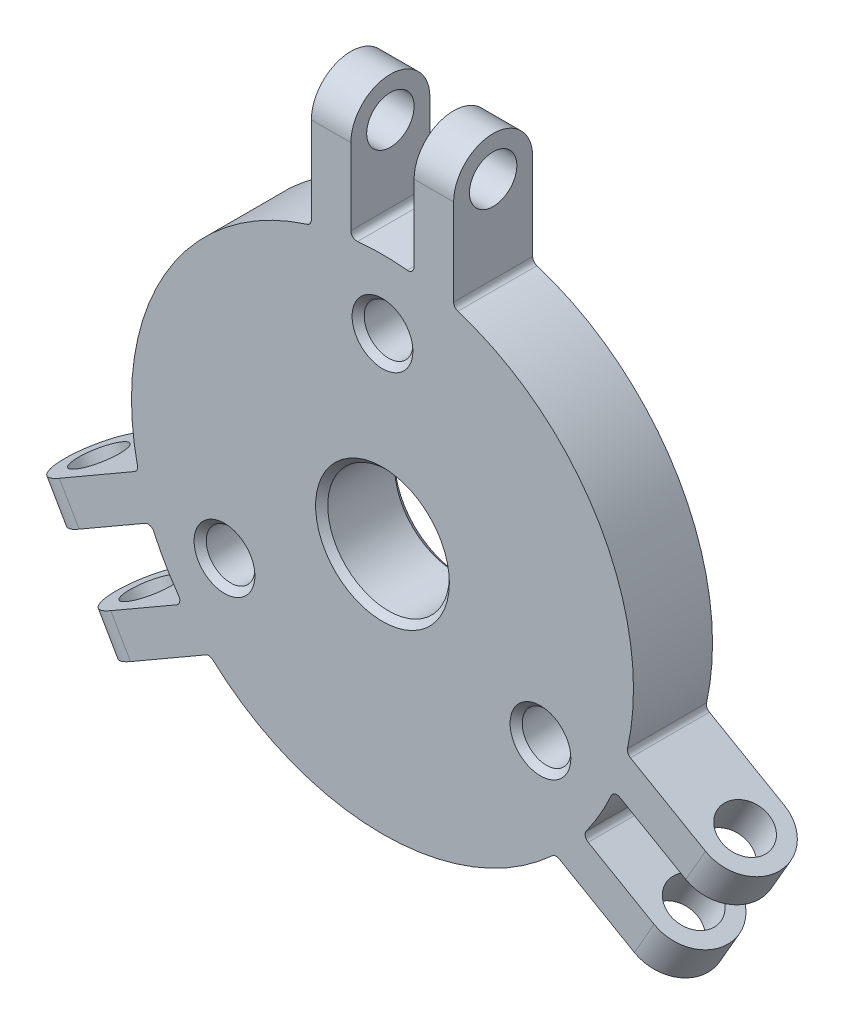
SolidWorks part; units mm, degrees
ref_plane "Front Plane" through (0, 0, 0) normal (0, 0, 1) x (1, 0, 0)
ref_plane "Top Plane" through (0, 0, 0) normal (0, 1, 0) x (1, 0, 0)
ref_plane "Right Plane" through (0, 0, 0) normal (1, 0, 0) x (0, 0, -1)
sketch "Sketch1" plane through (0, 0, 0) normal (0, 0, 1) x (1, 0, 0)
  line L0 (-27.5, -15.8771) -> (0, 0) construction
  line L1 (0, 31.7543) -> (-27.5, -15.8771) construction
  line L2 (-27.5, -15.8771) -> (27.5, -15.8771) construction
  line L3 (27.5, -15.8771) -> (0, 31.7543) construction
  line L4 (0, 0) -> (0, 31.7543) construction
  line L5 (0, 0) -> (27.5, -15.8771) construction
  line L6 (-26.5, -17.6092) -> (-12.6405, -9.6074)
  line L7 (-28.5, -14.1451) -> (-14.6405, -6.1433)
  line L8 (-29.75, -11.98) -> (-15.4362, -3.7159)
  line L9 (-25.25, -19.7742) -> (-10.9362, -11.5102)
  line L10 (-29.75, -11.98) -> (-15.8905, -3.9782) construction
  line L11 (-25.25, -19.7742) -> (-11.3905, -11.7724) construction
  line L12 (2, 31.7543) -> (2, 15.7507)
  line L13 (4.5, 31.7543) -> (4.5, 15.2261)
  line L14 (-29.75, -11.98) -> (-28.5, -14.1451)
  line L15 (-26.5, -17.6092) -> (-25.25, -19.7742)
  line L16 (4.5, 31.7543) -> (2, 31.7543)
  line L17 (-4.5, 31.7543) -> (-4.5, 15.2261)
  line L18 (-28.5, -14.1451) -> (-1, 1.7321) construction
  line L19 (-2, 31.7543) -> (-4.5, 31.7543)
  line L20 (-26.5, -17.6092) -> (1, -1.7321) construction
  line L21 (-2, 31.7543) -> (-2, 15.7507)
  line L22 (26.5, -17.6092) -> (12.6405, -9.6074)
  line L23 (25.25, -19.7742) -> (10.9362, -11.5102)
  line L24 (25.25, -19.7742) -> (26.5, -17.6092)
  line L25 (29.75, -11.98) -> (15.4362, -3.7159)
  line L26 (28.5, -14.1451) -> (29.75, -11.98)
  line L27 (28.5, -14.1451) -> (14.6405, -6.1433)
  circle A0 centre (0, 0) radius 15.8771 construction
  arc A1 (-14.6405, -6.1433) -> (-12.6405, -9.6074) centre (0, 0) ccw
  arc A2 (-10.9362, -11.5102) -> (10.9362, -11.5102) centre (0, 0) ccw
  arc A3 (2, 15.7507) -> (-2, 15.7507) centre (0, 0) ccw
  arc A4 (-4.5, 15.2261) -> (-15.4362, -3.7159) centre (0, 0) ccw
  arc A5 (15.4362, -3.7159) -> (4.5, 15.2261) centre (0, 0) ccw
  arc A6 (12.6405, -9.6074) -> (14.6405, -6.1433) centre (0, 0) ccw
  point P10 (1.5, 0)
  point P11 (1.5, 14.6647)
  point P12 (-1.5, 0)
  point P13 (-1.5, 14.6647)
  point P14 (-0.75, -1.299)
  point P15 (11.95, -8.6314)
  point P16 (0.75, 1.299)
  point P17 (13.45, -6.0333)
  point P44 (0, 0)
  dimension "D1" = 55
  dimension "D4" = 2.5
  dimension "D2" = 2
  dimension "D3" = 2
  dimension "D5" = 2.5
  dimension "D6" = 3
extrude "Boss-Extrude1" add sketch "Sketch1" along normal blind 5
sketch "Sketch2" plane through (0, 0, 0) normal (1, 0, 0) x (0, 0, -1)
  line L0 (-2.5, 31.7543) -> (-2.5, 22.1951) construction
  line L1 (-5, 31.7543) -> (0, 31.7543) construction
  circle A0 centre (-2.5, 21) radius 1.5
  dimension "D2" = 3
  dimension "D1" = 21
extrude "Cut-Extrude1" cut sketch "Sketch2" against normal mid plane 31
sketch "Sketch3" plane through (0, 0, 5) normal (0, 0, 1) x (1, 0, 0)
  circle A0 centre (0, 0) radius 7.5
  dimension "D1" = 15
extrude "Cut-Extrude2" [suppressed] cut sketch "Sketch3" against normal blind 8
sketch "Sketch4" plane through (-4.5, 0, 0) normal (-1, 0, 0) x (0, 0, 1)
  line L0 (0, 21) -> (0, 31.7543)
  line L1 (0, 31.7543) -> (5, 31.7543)
  line L2 (5, 31.7543) -> (5, 21)
  arc A0 (5, 21) -> (0, 21) centre (2.5, 21) ccw
extrude "Cut-Extrude3" cut sketch "Sketch4" against normal blind 27
pattern_circular "CirPattern1" count 3 over 360 about axis through (0, 0, 5) along (0, 0, -1) of "Cut-Extrude3"
pattern_circular "CirPattern2" count 3 over 360 about axis through (0, 0, 5) along (0, 0, -1) of "Cut-Extrude1"
scale "Scale ratio 1" scale about centroid uniform scaling yes scale factor 1.3
sketch "Sketch5" plane through (0, 0, 5.75) normal (0, 0, 1) x (1, 0, 0)
  circle A0 centre (0, 0) radius 5
  dimension "D1" = 10
extrude "Cut-Extrude4" cut sketch "Sketch5" against normal blind 10
chamfer "Chamfer1" distance 0.5 angle 45 2 edges at (5, 0, -0.75) (5, 0, 5.75)
ref_plane "Plane1" through (0, 0, 6.75) normal (0, 0, 1) x (1, 0, 0)
sketch "Sketch6" plane through (0, 0, 6.75) normal (0, 0, 1) x (1, 0, 0)
  circle A0 centre (0, 0) radius 8
  dimension "D1" = 16
sketch "Sketch8" plane through (0, 0, 5.75) normal (0, 0, 1) x (1, 0, 0)
  circle A0 centre (0, 15) radius 2
  circle A1 centre (12.9904, -7.5) radius 2
  circle A2 centre (-12.9904, -7.5) radius 2
  point P9 (0, 0)
  dimension "D2" = 4
  dimension "D1" = 15
  dimension "D3" = 3
extrude "Cut-Extrude5" cut sketch "Sketch8" against normal blind 10
chamfer "Chamfer2" distance 0.5 angle 45 6 edges at (14.9904, -7.5, -0.75) (14.9904, -7.5, 5.75) (-10.9904, -7.5, -0.75) (-10.9904, -7.5, 5.75) (2, 15, -0.75) (2, 15, 5.75)
fillet "Fillet1" radius 0.5 12 edges at (20.067, -4.8307, 2.5) (16.4326, -12.4896, 2.5) (19.0326, -7.9863, 2.5) (14.217, -14.9632, 2.5) (-16.4326, -12.4896, 2.5) (-14.217, -14.9632, 2.5) (-19.0326, -7.9863, 2.5) (-20.067, -4.8307, 2.5) (-5.85, 19.7939, 2.5) (-2.6, 20.4759, 2.5) (2.6, 20.4759, 2.5) (5.85, 19.7939, 2.5)
